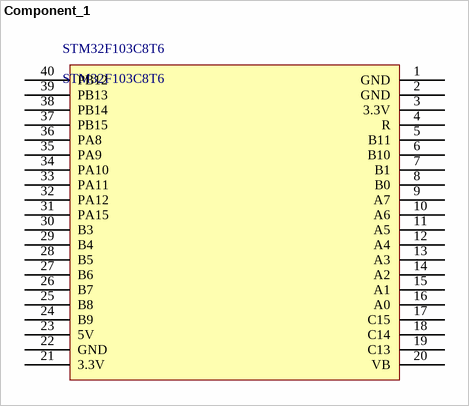
[diagram p0: symbol Component_1]
# Altium schematic symbol library MISC80722-7.SchLib: 1 symbol
Pins are listed as number, name and electrical type; pins without a type are passive.


## Component_1
designator STM32F103C8T6, comment STM32F103C8T6
footprint PCBComponent_1
pins: 1 GND (power), 2 GND (power), 3 3.3V (power), 4 R, 5 B11, 6 B10, 7 B1, 8 B0, 9 A7, 10 A6, 11 A5, 12 A4, 13 A3, 14 A2, 15 A1, 16 A0, 17 C15, 18 C14, 19 C13, 20 VB, 21 3.3V (power), 22 GND (power), 23 5V (power), 24 B9, 25 B8, 26 B7, 27 B6, 28 B5, 29 B4, 30 B3, 31 PA15, 32 PA12, 33 PA11, 34 PA10, 35 PA9, 36 PA8, 37 PB15, 38 PB14, 39 PB13, 40 PB12